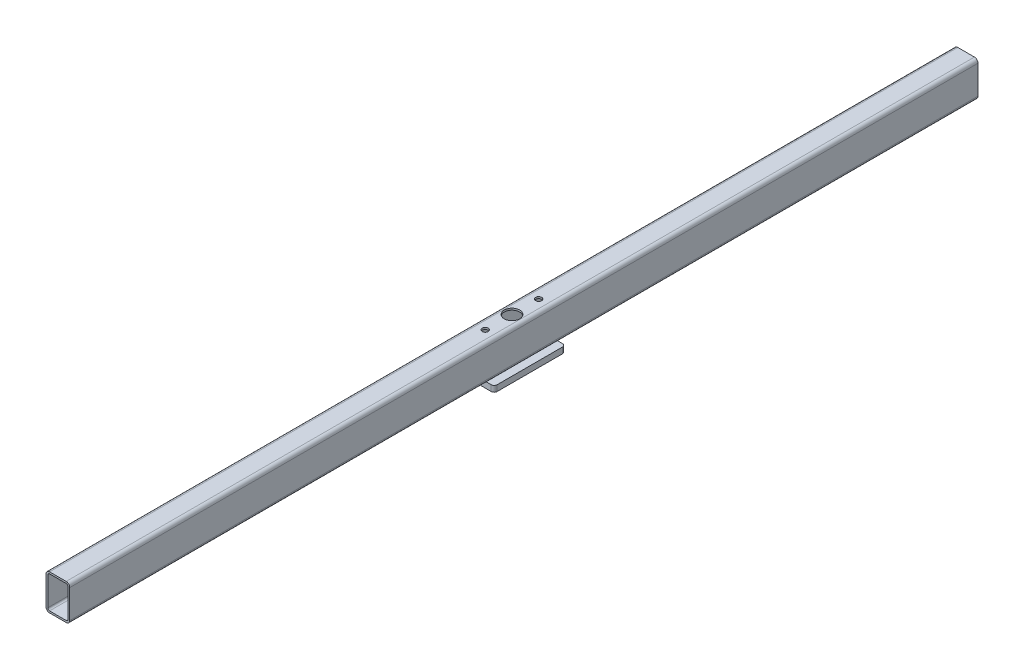
SolidWorks part; units mm, degrees
material "普通碳钢"
ref_plane "Front Plane" through (0, 0, 0) normal (0, 0, 1) x (1, 0, 0)
ref_plane "Top Plane" through (0, 0, 0) normal (0, 1, 0) x (1, 0, 0)
ref_plane "Right Plane" through (0, 0, 0) normal (1, 0, 0) x (0, 0, -1)
other "Configuration Table"
sketch "Sketch1" plane through (0, 0, 0) normal (0, 1, 0) x (1, 0, 0)
  line L0 (0, 0) -> (0, 1530)
  dimension "D1" = 1530
other "Gb/6728-1986 rectangular hollow section 060 X 40 X 3"
ref_plane "Plane1" through (0, 0, 0) normal (0, 0, -1) x (-1, 0, 0)
sketch "Sketch14" plane through (0, 0, 0) normal (0, 0, -1) x (-1, 0, 0)
  line L0 (-14, -27) -> (14, -27)
  line L1 (-17, -24) -> (-17, 24)
  line L2 (14, 27) -> (-14, 27)
  line L3 (17, 24) -> (17, -24)
  line L4 (-14, -30) -> (14, -30)
  line L5 (-20, -24) -> (-20, 24)
  line L6 (14, 30) -> (-14, 30)
  line L7 (20, 24) -> (20, -24)
  arc A0 (20, 24) -> (14, 30) centre (14, 24) ccw
  arc A1 (14, -30) -> (20, -24) centre (14, -24) ccw
  arc A2 (-20, -24) -> (-14, -30) centre (-14, -24) ccw
  arc A3 (-14, 30) -> (-20, 24) centre (-14, 24) ccw
  arc A4 (-14, 27) -> (-17, 24) centre (-14, 24) ccw
  arc A5 (17, 24) -> (14, 27) centre (14, 24) ccw
  arc A6 (14, -27) -> (17, -24) centre (14, -24) ccw
  arc A7 (-17, -24) -> (-14, -27) centre (-14, -24) ccw
  point P0 (0, 30)
  point P1 (20, 0)
  point P2 (0, -30)
  point P3 (-20, 0)
  point P4 (-20, 30)
  point P5 (20, 30)
  point P6 (20, -30)
  point P7 (-20, -30)
  point P8 (0, 0)
  point P33 (0, 0)
  dimension "D1" = 6
  dimension "Thickness" = 3
  dimension "V_leg" = 60
  dimension "H_leg" = 40
sketch "Sketch2" plane through (-20, 0, 0) normal (-1, 0, 0) x (0, 0, 1)
  line L0 (-1530, 0) -> (0, 0) construction
  line L1 (-1530, -24) -> (-1530, 24) construction
  circle A0 centre (-740, 0) radius 15
  dimension "D1" = 30
  dimension "D2" = 790
sketch "Sketch5" plane through (0, 30, 0) normal (0, 1, 0) x (1, 0, 0)
  line L0 (0, 0) -> (0, 1530) construction
  line L1 (-14, 1530) -> (14, 1530) construction
  circle A0 centre (0, 765) radius 13
  dimension "D1" = 26
  dimension "D2" = 765
extrude "Cut-Extrude1" cut sketch "Sketch5" against normal blind 214
sketch "Sketch6" plane through (0, -30, 0) normal (0, -1, 0) x (1, 0, 0)
  line L1 (-30, -825) -> (30, -825)
  line L2 (-30, -825) -> (-30, -705)
  line L3 (-30, -705) -> (30, -705)
  line L4 (30, -825) -> (30, -705)
  line L5 (-30, -825) -> (30, -705) construction
  line L6 (-30, -705) -> (30, -825) construction
  line L7 (0, -715) -> (0, -725) construction
  line L8 (0, 0) -> (0, -1530) construction
  line L9 (4.5, -715) -> (4.5, -725)
  line L10 (-4.5, -715) -> (-4.5, -725)
  line L11 (0, -805) -> (0, -815) construction
  line L12 (4.5, -805) -> (4.5, -815)
  line L13 (-4.5, -805) -> (-4.5, -815)
  circle A0 centre (0, -765) radius 13
  arc A1 (4.5, -715) -> (-4.5, -715) centre (0, -715) ccw
  arc A2 (-4.5, -725) -> (4.5, -725) centre (0, -725) ccw
  arc A3 (4.5, -805) -> (-4.5, -805) centre (0, -805) ccw
  arc A4 (-4.5, -815) -> (4.5, -815) centre (0, -815) ccw
  point P0 (0, -765)
  point P14 (0, -720)
  point P21 (0, -810)
  dimension "D8" = 26
  dimension "D1" = 120
  dimension "D2" = 9
  dimension "D3" = 10
  dimension "D4" = 45
  dimension "D5" = 9
  dimension "D6" = 10
  dimension "D7" = 45
  dimension "D9" = 60
extrude "Boss-Extrude1" add sketch "Sketch6" along normal blind 10 separate body
sketch "Sketch7" plane through (0, -30, 0) normal (0, -1, 0) x (1, 0, 0)
  line L0 (0, 0) -> (0, -1530) construction
  line L1 (-4.5, -810) -> (4.5, -810) construction
  line L2 (-4.5, -805) -> (-4.5, -815) construction
  line L3 (4.5, -815) -> (4.5, -805) construction
  line L5 (0, -705) -> (0, -825) construction
  line L6 (30, -705) -> (-30, -705) construction
  line L7 (-30, -825) -> (30, -825) construction
  circle A0 centre (0, -720) radius 5
  circle A1 centre (0, -810) radius 5
  circle A3 centre (0, -765) radius 13 construction
  dimension "D1" = 10
  dimension "D2" = 10
  dimension "D3" = 45
extrude "Cut-Extrude2" cut sketch "Sketch7" against normal through all
fillet "Fillet1" radius 5 4 edges at (-30, -35, -825) (30, -35, -825) (30, -35, -705) (-30, -35, -705)
